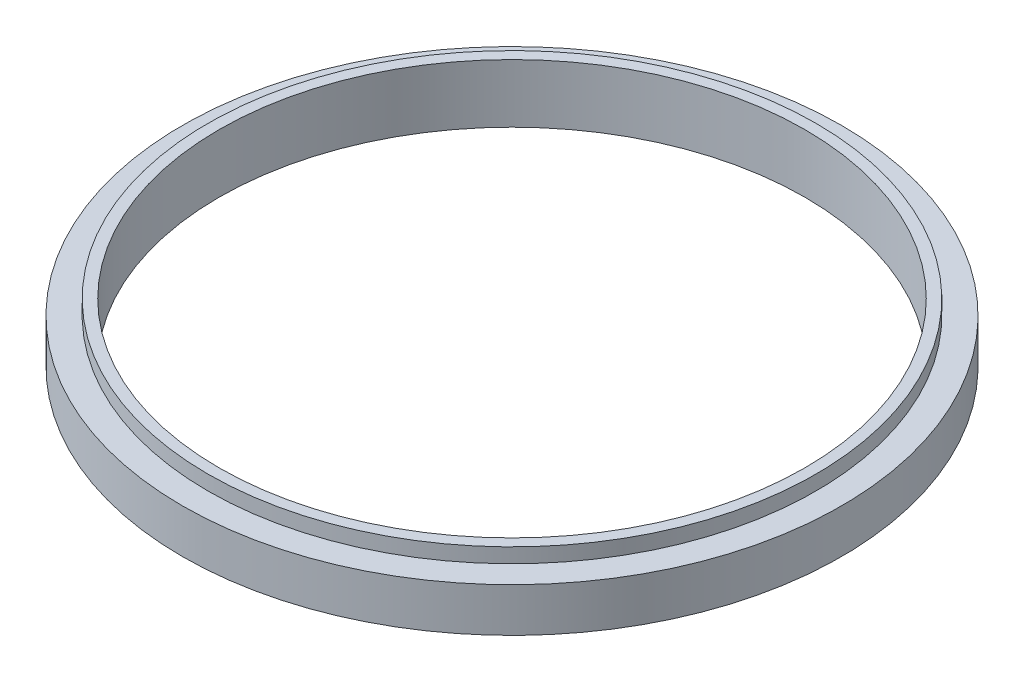
from build123d import *

# Parameters (mm, degrees)
SKETCH1_R           = 45
SKETCH1_R_2         = 40
BOSS_EXTRUDE1_DEPTH = 6
SKETCH2_R           = 41.5
SKETCH2_R_2         = 40
BOSS_EXTRUDE2_DEPTH = 2


with BuildPart() as part:
    # Sketch1 → Boss-Extrude1 (new body)
    with BuildSketch(Plane(origin=(0, 0, 0), x_dir=(1, 0, 0), z_dir=(0, 1, 0))):
        with Locations(Location((0, 0, 0), (0, 0, 270))):
            Circle(SKETCH1_R)
        with Locations(Location((0, 0, 0), (0, 0, 270))):
            Circle(SKETCH1_R_2, mode=Mode.SUBTRACT)
    extrude(amount=BOSS_EXTRUDE1_DEPTH)

    # Sketch2 → Boss-Extrude2 (add)
    with BuildSketch(Plane(origin=(0, 6, 0), x_dir=(1, 0, 0), z_dir=(0, 1, 0))):
        with Locations(Location((0, 0, 0), (0, 0, 270))):
            Circle(SKETCH2_R)
        with Locations(Location((0, 0, 0), (0, 0, 270))):
            Circle(SKETCH2_R_2, mode=Mode.SUBTRACT)
    extrude(amount=BOSS_EXTRUDE2_DEPTH)


solid = part.part
